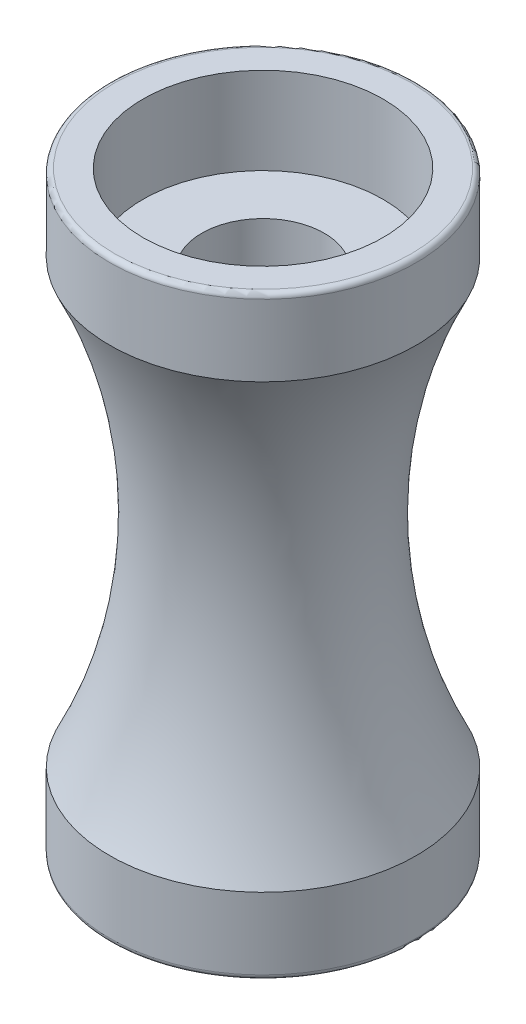
from build123d import *

# Parameters (mm, degrees)
SKETCH_2_R          = 12
CUT_EXTRUDE_1_DEPTH = 116.5
SKETCH_3_R          = 23.5
SKETCH_3_R_2        = 10
CUT_EXTRUDE_2_DEPTH = 17
CUT_EXTRUDE_START   = -17
SKETCH_4_R          = 23.5
SKETCH_4_R_2        = 10
CUT_EXTRUDE_3_DEPTH = 17
FILLET_1_R          = 1


with BuildPart() as part:
    # 草图1 → 旋转1 (revolve)
    with BuildSketch(Plane.XY, mode=Mode.PRIVATE) as revolve_1_sk:
        with BuildLine():
            Line((0, 0), (0, 116.5))
            Line((0, 116.5), (30, 116.5))
            Line((30, 116.5), (30, 101.5))
            ThreePointArc((30, 101.5), (20, 58.25), (30, 15))
            Line((30, 15), (30, 0))
            Line((30, 0), (0, 0))
        make_face()
    revolve(revolve_1_sk.sketch.rotate(Axis((0, 0, 0), (0, 1, 0)), 90), axis=Axis((0, 0, 0), (0, 1, 0)))

    # 草图2 → 切除-拉伸1 (cut)
    with BuildSketch(Plane(origin=(0, 116.5, 0), x_dir=(1, 0, 0), z_dir=(0, 1, 0))):
        with Locations(Location((0, 0, 0), (0, 0, 270))):
            Circle(SKETCH_2_R)
    extrude(amount=-CUT_EXTRUDE_1_DEPTH, mode=Mode.SUBTRACT)

    # 草图3 → 切除-拉伸2 (cut)
    with BuildSketch(Plane(origin=(0, 116.5, 0), x_dir=(1, 0, 0), z_dir=(0, 1, 0))):
        with Locations(Location((0, 0, 0), (0, 0, 270))):
            Circle(SKETCH_3_R)
        Circle(SKETCH_3_R_2, mode=Mode.SUBTRACT)
    extrude(amount=-CUT_EXTRUDE_2_DEPTH, mode=Mode.SUBTRACT)

    # 草图4 → 切除-拉伸3 (cut)
    with BuildSketch(Plane.XZ.offset(CUT_EXTRUDE_START)):
        with Locations(Location((0, 0, 0), (0, 0, 90))):
            Circle(SKETCH_4_R)
        Circle(SKETCH_4_R_2, mode=Mode.SUBTRACT)
    extrude(amount=CUT_EXTRUDE_3_DEPTH, mode=Mode.SUBTRACT)

    # 圆角1
    fillet_1_edges = [part.edges().sort_by_distance(p)[0] for p in [
        (0, 116.5, 30),
        (0, 0, 30),
    ]]
    fillet(fillet_1_edges, radius=FILLET_1_R)


solid = part.part
